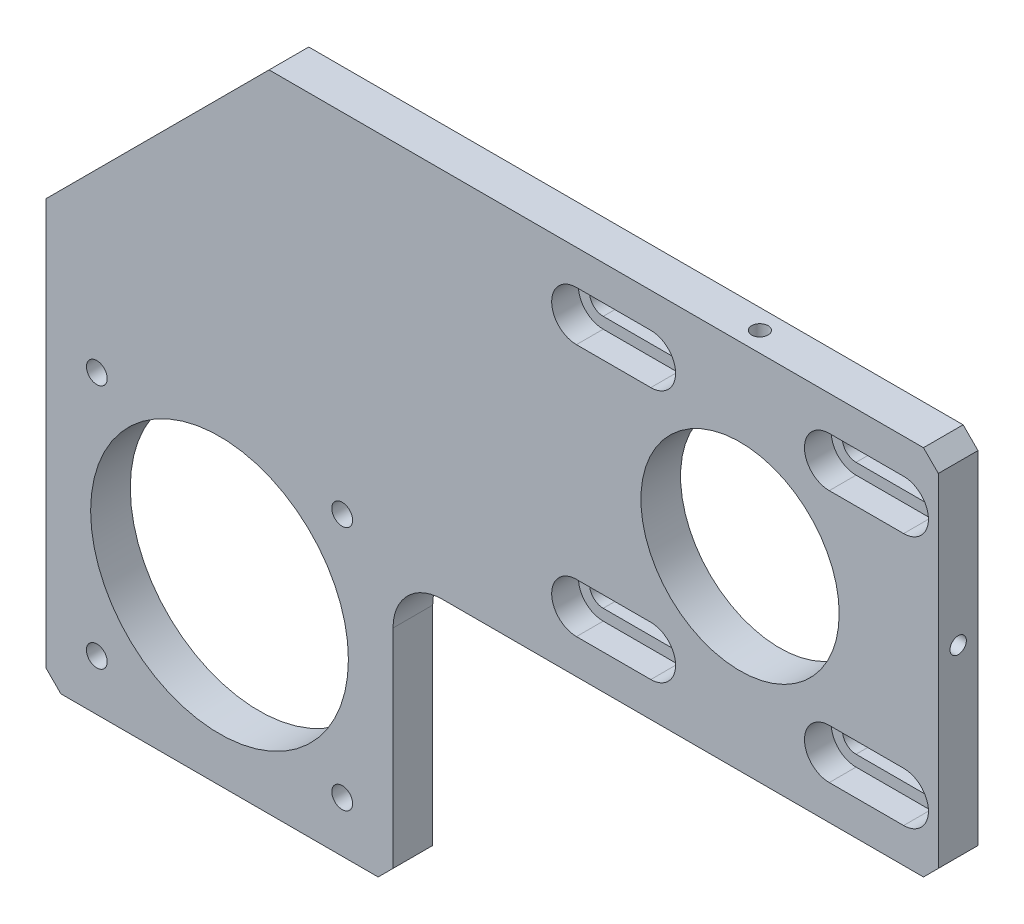
SolidWorks part; units mm, degrees
ref_plane "前视基准面" through (0, 0, 0) normal (0, 0, 1) x (1, 0, 0)
ref_plane "上视基准面" through (0, 0, 0) normal (0, 1, 0) x (1, 0, 0)
ref_plane "右视基准面" through (0, 0, 0) normal (1, 0, 0) x (0, 0, -1)
sketch "草图2" plane through (0, 0, 0) normal (0, 0, 1) x (1, 0, 0)
  line L1 (-90, 65) -> (90, 65)
  line L2 (-90, 65) -> (-90, -65)
  line L3 (-90, -65) -> (90, -65)
  line L4 (90, 65) -> (90, -65)
  line L5 (-90, 65) -> (90, -65) construction
  line L6 (-90, -65) -> (90, 65) construction
  point P0 (0, 0)
  dimension "D1" = 180
  dimension "D2" = 130
extrude "凸台-拉伸1" add sketch "草图2" along normal mid plane 8
sketch "草图3" plane through (0, 0, 4) normal (0, 0, 1) x (1, 0, 0)
  line L0 (-90, 65) -> (-90, -65) construction
  line L1 (90, -65) -> (-20, -65)
  line L2 (90, -65) -> (90, -10)
  line L3 (90, -10) -> (-20, -10)
  line L4 (-20, -65) -> (-20, -10)
  line L5 (90, 65) -> (-90, 65) construction
  dimension "D1" = 70
  dimension "D2" = 75
extrude "切除-拉伸1" cut sketch "草图3" against normal blind 8
sketch "草图4" plane through (0, 0, 4) normal (0, 0, 1) x (1, 0, 0)
  line L0 (90, 65) -> (-90, 65) construction
  line L1 (-90, 65) -> (-90, -65) construction
  circle A0 centre (-55, -30) radius 26
  dimension "D1" = 95
  dimension "D2" = 35
  dimension "D3" = 52
extrude "切除-拉伸2" cut sketch "草图4" against normal blind 8
hole_wizard "M5 螺纹孔1" positions "草图6" profile "草图5" tap size "M5" standard "ISO"
sketch "草图6" plane through (0, 0, 4) normal (0, 0, 1) x (1, 0, 0)
  line L2 (-79.7487, -5.2513) -> (-30.2513, -5.2513)
  line L3 (-79.7487, -5.2513) -> (-79.7487, -54.7487)
  line L4 (-79.7487, -54.7487) -> (-30.2513, -54.7487)
  line L5 (-30.2513, -5.2513) -> (-30.2513, -54.7487)
  line L6 (-79.7487, -5.2513) -> (-30.2513, -54.7487) construction
  line L7 (-79.7487, -54.7487) -> (-30.2513, -5.2513) construction
  circle A0 centre (-55, -30) radius 35 construction
  point P8 (-30.2513, -54.7487)
  point P69 (-79.7487, -5.2513)
  point P70 (-79.7487, -54.7487)
  point P71 (-30.2513, -5.2513)
  dimension "D1" = 70
  dimension "D2" = 90
sketch "草图5" plane through (-30.2513, -54.7487, 4) normal (1, 0, 0) x (0, -1, 0)
  line L0 (0, 0) -> (0, 13.6618)
  line L1 (0, 13.6618) -> (2.1, 12.4)
  line L2 (2.1, 12.4) -> (2.1, 0)
  line L5 (2.1, 0) -> (0, 0)
  line L10 (0, 13.6618) -> (-2.1, 12.4) construction
  line L11 (0, -6.35) -> (0, 107.95) construction
  dimension "螺纹孔钻头直径" = 4.2
  dimension "螺纹孔钻头深度" = 12.4
  dimension "导头角度" = 118
cosmetic thread "孔螺蚊线1" parameters "D1"=8, "D2"=5
cosmetic thread "孔螺蚊线2" parameters "D1"=8, "D2"=5
cosmetic thread "孔螺蚊线3" parameters "D1"=8, "D2"=5
cosmetic thread "孔螺蚊线4" parameters "D1"=8, "D2"=5
sketch "草图7" plane through (0, 0, 4) normal (0, 0, 1) x (1, 0, 0)
  line L0 (90, 65) -> (-90, 65) construction
  line L1 (90, -10) -> (90, 65) construction
  circle A0 centre (50, 27.5) radius 20
  dimension "D1" = 40
  dimension "D3" = 40
  dimension "D2" = 37.5
extrude "切除-拉伸3" cut sketch "草图7" against normal blind 8
sketch "草图8" plane through (0, 0, 4) normal (0, 0, 1) x (1, 0, 0)
  line L0 (70.5, 2) -> (80.5, 2) construction
  line L1 (70.5, 10.6) -> (80.5, 10.6)
  line L2 (70.5, -6.6) -> (80.5, -6.6)
  line L3 (90, -10) -> (-20, -10) construction
  line L4 (90, -10) -> (90, 65) construction
  line L5 (90.0463, 27.5) -> (16.7131, 27.5) construction
  line L6 (70.5, 53) -> (80.5, 53) construction
  line L7 (70.5, 44.4) -> (80.5, 44.4)
  line L8 (70.5, 61.6) -> (80.5, 61.6)
  line L9 (19.5, 2) -> (29.5, 2) construction
  line L10 (19.5, 10.6) -> (29.5, 10.6)
  line L11 (19.5, -6.6) -> (29.5, -6.6)
  line L12 (19.5, 53) -> (29.5, 53) construction
  line L13 (19.5, 44.4) -> (29.5, 44.4)
  line L14 (19.5, 61.6) -> (29.5, 61.6)
  arc A0 (70.5, 10.6) -> (70.5, -6.6) centre (70.5, 2) ccw
  arc A1 (80.5, -6.6) -> (80.5, 10.6) centre (80.5, 2) ccw
  arc A2 (70.5, 44.4) -> (70.5, 61.6) centre (70.5, 53) cw
  arc A3 (80.5, 61.6) -> (80.5, 44.4) centre (80.5, 53) cw
  arc A4 (19.5, 10.6) -> (19.5, -6.6) centre (19.5, 2) ccw
  arc A5 (29.5, -6.6) -> (29.5, 10.6) centre (29.5, 2) ccw
  arc A6 (19.5, 44.4) -> (19.5, 61.6) centre (19.5, 53) cw
  arc A7 (29.5, 61.6) -> (29.5, 44.4) centre (29.5, 53) cw
  point P2 (75.5, 2)
  point P16 (75.5, 53)
  point P25 (24.5, 2)
  point P32 (24.5, 53)
  dimension "D3" = 12
  dimension "D4" = 9.5
  dimension "D1" = 10
  dimension "D2" = 17.2
  dimension "D5" = 2
extrude "切除-拉伸4" [suppressed] cut sketch "草图8" against normal blind 6
sketch "草图9" [suppressed] plane through (0, 0, -2) normal (0, 0, 1) x (1, 0, 0)
  line L0 (70.5, 2) -> (80.5, 2) construction
  line L1 (70.5, 5.3) -> (80.5, 5.3)
  line L2 (70.5, -1.3) -> (80.5, -1.3)
  line L3 (87.6587, 27.5) -> (3.2403, 27.5) construction
  line L4 (70.5, 53) -> (80.5, 53) construction
  line L5 (70.5, 49.7) -> (80.5, 49.7)
  line L6 (70.5, 56.3) -> (80.5, 56.3)
  line L7 (19.5, 2) -> (29.5, 2) construction
  line L8 (19.5, 5.3) -> (29.5, 5.3)
  line L9 (19.5, -1.3) -> (29.5, -1.3)
  line L10 (19.5, 53) -> (29.5, 53) construction
  line L11 (19.5, 49.7) -> (29.5, 49.7)
  line L12 (19.5, 56.3) -> (29.5, 56.3)
  arc A0 (70.5, 5.3) -> (70.5, -1.3) centre (70.5, 2) ccw
  arc A1 (80.5, -1.3) -> (80.5, 5.3) centre (80.5, 2) ccw
  arc A2 (70.5, 49.7) -> (70.5, 56.3) centre (70.5, 53) cw
  arc A3 (80.5, 56.3) -> (80.5, 49.7) centre (80.5, 53) cw
  arc A4 (19.5, 5.3) -> (19.5, -1.3) centre (19.5, 2) ccw
  arc A5 (29.5, -1.3) -> (29.5, 5.3) centre (29.5, 2) ccw
  arc A6 (19.5, 49.7) -> (19.5, 56.3) centre (19.5, 53) cw
  arc A7 (29.5, 56.3) -> (29.5, 49.7) centre (29.5, 53) cw
  point P3 (75.5, 2)
  point P13 (75.5, 53)
  point P22 (24.5, 2)
  point P29 (24.5, 53)
  dimension "D2" = 3.3
  dimension "D1" = 10
  dimension "D3" = 2
extrude "切除-拉伸5" [suppressed] cut sketch "草图9" against normal blind 6
hole_wizard "M4 螺纹孔1" positions "草图11" profile "草图10" tap size "M4" standard "ISO"
sketch "草图11" plane through (0, 65, 0) normal (0, 1, 0) x (1, 0, 0)
  line L0 (90, -4) -> (90, 4) construction
  point P0 (50, 0)
  dimension "D1" = 40
sketch "草图10" plane through (50, 65, 0) normal (1, 0, 0) x (0, 0, 1)
  line L0 (0, 0) -> (0, 12.9914)
  line L1 (0, 12.9914) -> (1.65, 12)
  line L2 (1.65, 12) -> (1.65, 0)
  line L5 (1.65, 0) -> (0, 0)
  line L10 (0, 12.9914) -> (-1.65, 12) construction
  line L11 (0, -6.35) -> (0, 107.95) construction
  dimension "螺纹孔钻头直径" = 3.3
  dimension "螺纹孔钻头深度" = 12
  dimension "导头角度" = 118
cosmetic thread "孔螺蚊线5" parameters "D1"=8, "D2"=4
hole_wizard "M4 螺纹孔2" positions "草图13" profile "草图12" tap size "M4" standard "ISO"
sketch "草图13" plane through (0, -65, 0) normal (0, -1, 0) x (-1, 0, 0)
  line L0 (-90, 4) -> (-90, -4) construction
  point P0 (40, 0)
  dimension "D1" = 130
sketch "草图12" plane through (-40, -65, 0) normal (1, 0, 0) x (0, 0, -1)
  line L0 (0, 0) -> (0, 12.9914)
  line L1 (0, 12.9914) -> (1.65, 12)
  line L2 (1.65, 12) -> (1.65, 0)
  line L5 (1.65, 0) -> (0, 0)
  line L10 (0, 12.9914) -> (-1.65, 12) construction
  line L11 (0, -6.35) -> (0, 107.95) construction
  dimension "螺纹孔钻头直径" = 3.3
  dimension "螺纹孔钻头深度" = 12
  dimension "导头角度" = 118
cosmetic thread "孔螺蚊线6" parameters "D1"=8, "D2"=4
chamfer "倒角1" distance 45 angle 45 1 edges at (-90, 65, 0)
chamfer "倒角2" distance 3 angle 45 4 edges at (-90, -65, 0) (-20, -65, 0) (90, -10, 0) (90, 65, 0)
fillet "圆角1" radius 10 1 edges at (-20, -10, 0)
hole_wizard "M6 六角凹头螺钉的柱形沉头孔1" positions "草图15" profile "草图14" counterbore size "M6" standard "ISO"
sketch "草图15" plane through (0, 0, 4) normal (0, 0, 1) x (1, 0, 0)
  point P0 (-21.5202, 50.3478)
sketch "草图14" plane through (-21.5202, 50.3478, 4) normal (1, 0, 0) x (0, -1, 0)
  line L0 (0, 0) -> (0, 12.0828)
  line L1 (0, 12.0828) -> (3.3, 10.1)
  line L2 (3.3, 10.1) -> (3.3, 6.4)
  line L3 (3.3, 6.4) -> (5.5, 6.4)
  line L4 (5.5, 6.4) -> (5.5, 0)
  line L5 (5.5, 0) -> (0, 0)
  line L10 (0, 12.0828) -> (-3.3, 10.1) construction
  line L11 (0, -6.35) -> (0, 107.95) construction
  dimension "孔直径" = 6.6
  dimension "孔深度" = 10.1
  dimension "柱形沉头孔直径" = 11
  dimension "柱形沉头孔深度" = 6.4
  dimension "导头角度" = 118
hole_wizard "M5 六角凹头螺钉的柱形沉头孔1" positions "草图17" profile "草图16" counterbore size "M5" standard "ISO"
sketch "草图17" plane through (0, 0, 4) normal (0, 0, 1) x (1, 0, 0)
  line L0 (50, 27.5) -> (50, 71.9229) construction
  line L2 (50, 27.5) -> (108.5646, 27.5) construction
  point P0 (24.5, 53)
  point P2 (75.5, 53)
  point P4 (24.5, 2)
  point P6 (75.5, 2)
  dimension "D1" = 51
  dimension "D2" = 51
sketch "草图16" plane through (24.5, 53, 4) normal (1, 0, 0) x (0, -1, 0)
  line L0 (0, 0) -> (0, 11.7524)
  line L1 (0, 11.7524) -> (2.75, 10.1)
  line L2 (2.75, 10.1) -> (2.75, 5.4)
  line L3 (2.75, 5.4) -> (5, 5.4)
  line L4 (5, 5.4) -> (5, 0)
  line L5 (5, 0) -> (0, 0)
  line L10 (0, 11.7524) -> (-2.75, 10.1) construction
  line L11 (0, -6.35) -> (0, 107.95) construction
  dimension "孔直径" = 5.5
  dimension "孔深度" = 10.1
  dimension "柱形沉头孔直径" = 10
  dimension "柱形沉头孔深度" = 5.4
  dimension "导头角度" = 118
sketch "草图18" plane through (0, 0, 4) normal (0, 0, 1) x (1, 0, 0)
  line L0 (17, 53) -> (32, 53) construction
  line L1 (17, 55.75) -> (32, 55.75)
  line L2 (17, 50.25) -> (32, 50.25)
  arc A0 (17, 55.75) -> (17, 50.25) centre (17, 53) ccw
  arc A1 (32, 50.25) -> (32, 55.75) centre (32, 53) ccw
  circle A2 centre (24.5, 53) radius 2.75 construction
  point P2 (24.5, 53)
  dimension "D1" = 15
extrude "切除-拉伸6" cut sketch "草图18" against normal through all
sketch "草图19" plane through (0, 0, 4) normal (0, 0, 1) x (1, 0, 0)
  line L0 (17, 53) -> (32, 53) construction
  line L1 (17, 58) -> (32, 58)
  line L2 (17, 48) -> (32, 48)
  arc A0 (17, 58) -> (17, 48) centre (17, 53) ccw
  arc A1 (32, 48) -> (32, 58) centre (32, 53) ccw
  arc A2 (28.6758, 55.75) -> (20.3242, 55.75) centre (24.5, 53) ccw construction
  point P2 (24.5, 53)
extrude "切除-拉伸7" cut sketch "草图19" against normal up to surface (5.4 mm away) up to face at (24.5, 56.875, -1.4)
pattern_linear "阵列(线性)1" count 2 spacing 51 along (1, 0, 0) count 2 spacing 51 along (0, -1, 0) of "切除-拉伸6", "切除-拉伸7"
hole_wizard "M4 螺纹孔3" positions "草图21" profile "草图20" tap size "M4" standard "ISO"
sketch "草图21" plane through (-90, 0, 0) normal (-1, 0, 0) x (0, 0, 1)
  line L0 (4, -65) -> (-4, -65) construction
  point P0 (0, -15)
  dimension "D1" = 50
sketch "草图20" plane through (-90, -15, 0) normal (0, 1, 0) x (0, 0, 1)
  line L0 (0, 0) -> (0, 11.0914)
  line L1 (0, 11.0914) -> (1.65, 10.1)
  line L2 (1.65, 10.1) -> (1.65, 0)
  line L5 (1.65, 0) -> (0, 0)
  line L10 (0, 11.0914) -> (-1.65, 10.1) construction
  line L11 (0, -6.35) -> (0, 107.95) construction
  dimension "螺纹孔钻头直径" = 3.3
  dimension "螺纹孔钻头深度" = 10.1
  dimension "导头角度" = 118
cosmetic thread "孔螺蚊线7" parameters "D1"=8, "D2"=4
hole_wizard "M4 螺纹孔4" positions "草图23" profile "草图22" tap size "M4" standard "ISO"
sketch "草图23" plane through (90, 0, 0) normal (1, 0, 0) x (0, 0, -1)
  line L0 (4, -10) -> (-4, -10) construction
  point P0 (0, 30)
  dimension "D1" = 40
sketch "草图22" plane through (90, 30, 0) normal (0, 1, 0) x (0, 0, -1)
  line L0 (0, 0) -> (0, 11.0914)
  line L1 (0, 11.0914) -> (1.65, 10.1)
  line L2 (1.65, 10.1) -> (1.65, 0)
  line L5 (1.65, 0) -> (0, 0)
  line L10 (0, 11.0914) -> (-1.65, 10.1) construction
  line L11 (0, -6.35) -> (0, 107.95) construction
  dimension "螺纹孔钻头直径" = 3.3
  dimension "螺纹孔钻头深度" = 10.1
  dimension "导头角度" = 118
cosmetic thread "孔螺蚊线8" parameters "D1"=8, "D2"=4
